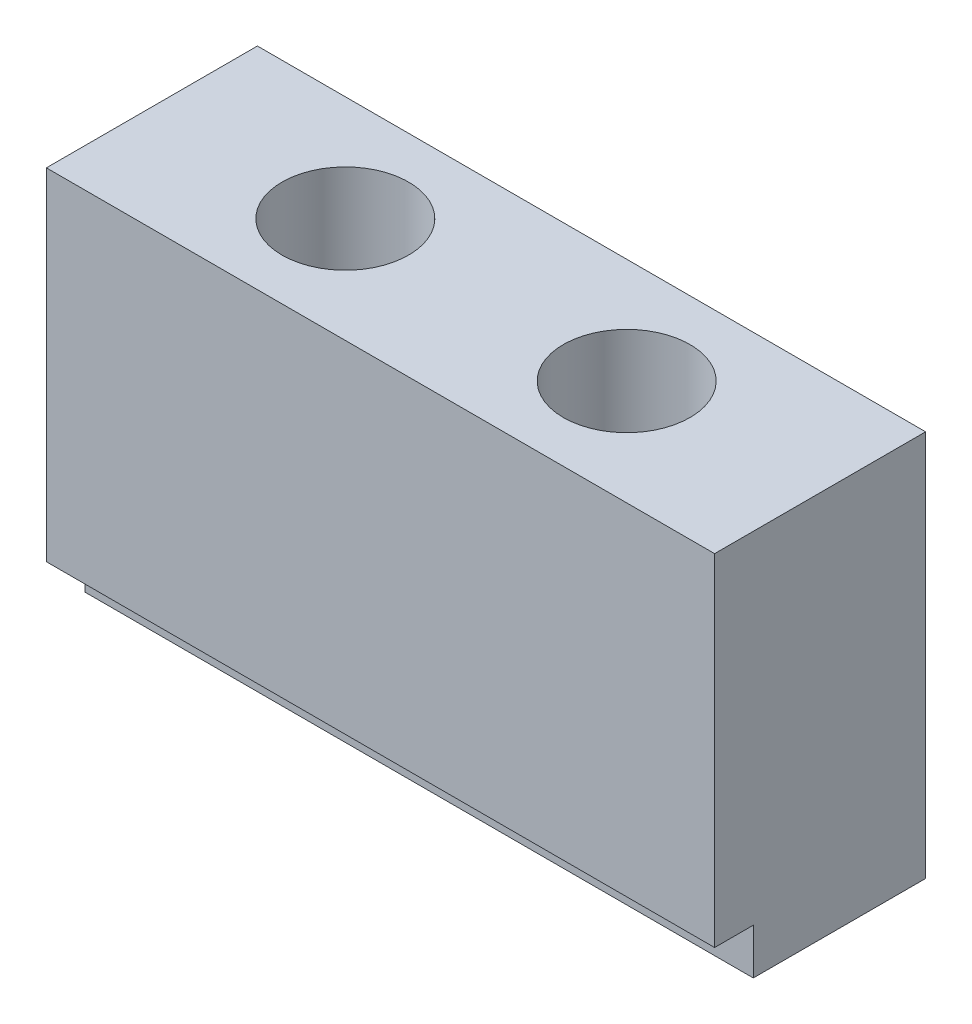
from build123d import *

# Parameters (mm, degrees)
SKETCH1_W           = 95
SKETCH1_H           = 30
BOSS_EXTRUDE1_DEPTH = 55
SKETCH2_R           = 5.5
CUT_EXTRUDE1_DEPTH  = 75.204110398
SKETCH3_R           = 9
CUT_EXTRUDE2_DEPTH  = 20
SKETCH4_W           = 5.5
SKETCH4_H           = 6.5
CUT_EXTRUDE3_DEPTH  = 172


with BuildPart() as part:
    # Sketch1 → Boss-Extrude1 (new body)
    with BuildSketch(Plane(origin=(0, 0, 0), x_dir=(1, 0, 0), z_dir=(0, 1, 0))):
        Rectangle(SKETCH1_W, SKETCH1_H)
    extrude(amount=BOSS_EXTRUDE1_DEPTH)

    # Sketch2 → Cut-Extrude1 (cut, through all)
    with BuildSketch(Plane(origin=(0, 55, 0), x_dir=(1, 0, 0), z_dir=(0, 1, 0))):
        with Locations(Location((-20, 0, 0), (0, 0, 270))):
            Circle(SKETCH2_R)
        with Locations(Location((20, 0, 0), (0, 0, 270))):
            Circle(SKETCH2_R)
    extrude(amount=-CUT_EXTRUDE1_DEPTH, mode=Mode.SUBTRACT)

    # Sketch3 → Cut-Extrude2 (cut)
    with BuildSketch(Plane(origin=(0, 55, 0), x_dir=(1, 0, 0), z_dir=(0, 1, 0))):
        with Locations(Location((-20, 0, 0), (0, 0, 270))):
            Circle(SKETCH3_R)
        with Locations(Location((20, 0, 0), (0, 0, 270))):
            Circle(SKETCH3_R)
    extrude(amount=-CUT_EXTRUDE2_DEPTH, mode=Mode.SUBTRACT)

    # Sketch4 → Cut-Extrude3 (cut)
    with BuildSketch(Plane.ZY.offset(47.5)):
        with Locations((12.25, 3.25)):
            Rectangle(SKETCH4_W, SKETCH4_H)
    extrude(amount=-CUT_EXTRUDE3_DEPTH, mode=Mode.SUBTRACT)


solid = part.part
